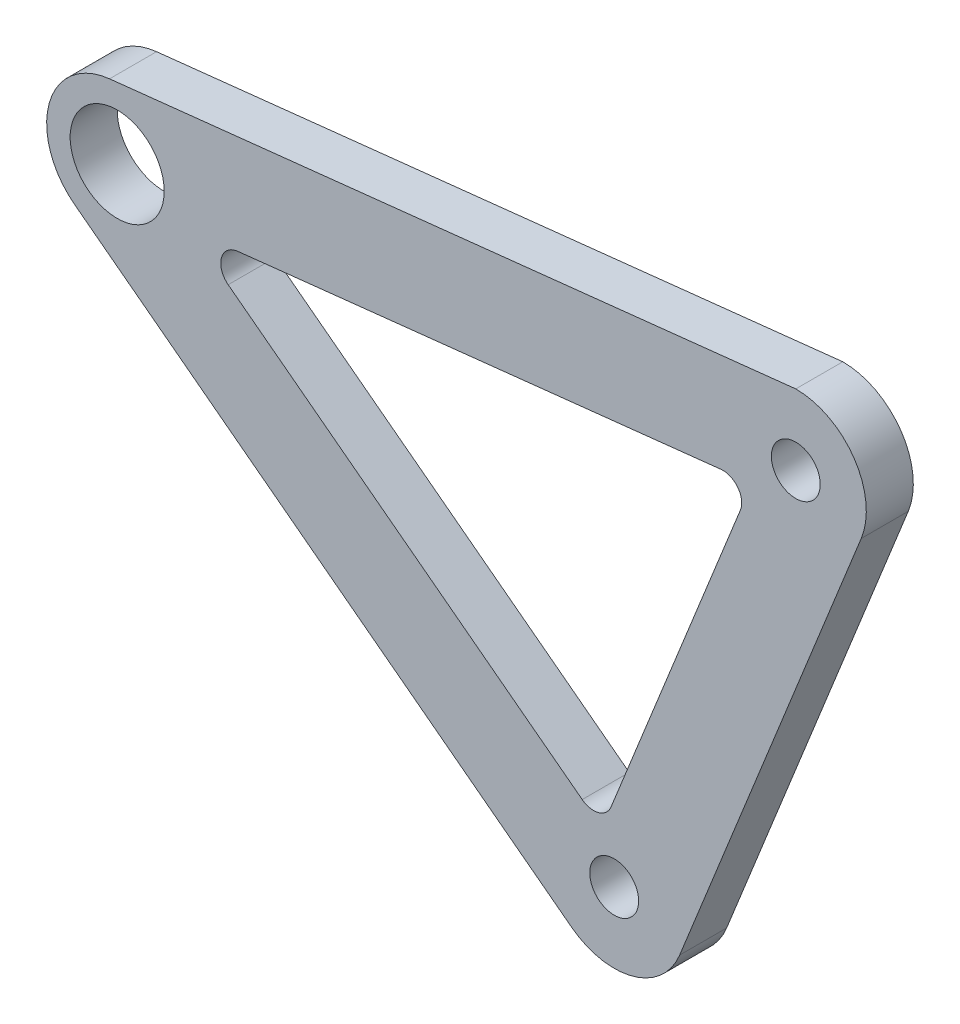
SolidWorks part; units mm, degrees
ref_plane "Front Plane" through (0, 0, 0) normal (0, 0, 1) x (1, 0, 0)
ref_plane "Top Plane" through (0, 0, 0) normal (0, 1, 0) x (1, 0, 0)
ref_plane "Right Plane" through (0, 0, 0) normal (1, 0, 0) x (0, 0, -1)
other "Configuration Table"
sketch "Sketch1" plane through (0, 0, 0) normal (0, 0, 1) x (1, 0, 0)
  line L0 (-72.1809, -7.8902) -> (-19.3137, -48.0361) construction
  line L1 (-19.3137, -48.0361) -> (0, 0) construction
  line L2 (0, 0) -> (-72.1809, -7.8902) construction
  line L3 (-72.9914, -0.4341) -> (0, 7.5)
  line L4 (-76.7167, -13.8632) -> (-23.8494, -54.0091)
  line L5 (6.9586, -2.7978) -> (-12.3551, -50.8339)
  line L6 (-7.9693, -3.889) -> (-59.3808, -9.5089)
  line L7 (-60.373, -13.0898) -> (-22.7179, -41.6841)
  line L8 (-19.6527, -40.8374) -> (-5.8964, -6.6233)
  line L9 (-20.6305, -43.2692) -> (-4.6512, -3.5263) construction
  line L10 (-64.3705, -10.0543) -> (-20.6305, -43.2692) construction
  line L11 (-4.6512, -3.5263) -> (-64.3705, -10.0543) construction
  circle A0 centre (0, 0) radius 2.6
  circle A1 centre (-19.3137, -48.0361) radius 2.6
  circle A2 centre (-72.1809, -7.8902) radius 5
  arc A3 (6.9586, -2.7978) -> (0, 7.5) centre (0, 0) ccw
  arc A4 (-23.8494, -54.0091) -> (-12.3551, -50.8339) centre (-19.3137, -48.0361) ccw
  arc A5 (-72.9914, -0.4341) -> (-76.7167, -13.8632) centre (-72.1809, -7.8902) ccw
  arc A6 (-19.6527, -40.8374) -> (-22.7179, -41.6841) centre (-21.5084, -40.0913) cw
  arc A7 (-5.8964, -6.6233) -> (-7.9693, -3.889) centre (-7.752, -5.8772) ccw
  arc A8 (-60.373, -13.0898) -> (-59.3808, -9.5089) centre (-59.1635, -11.497) cw
  dimension "D5" = 5.2
  dimension "D6" = 15
  dimension "D8" = 2
  dimension "D9" = 10
  dimension "D1" = 48.0361
  dimension "D2" = 19.3137
  dimension "D3" = 72.1809
  dimension "D4" = 7.8902
  dimension "D7" = 3
extrude "Boss-Extrude1" add sketch "Sketch1" along normal blind 5
